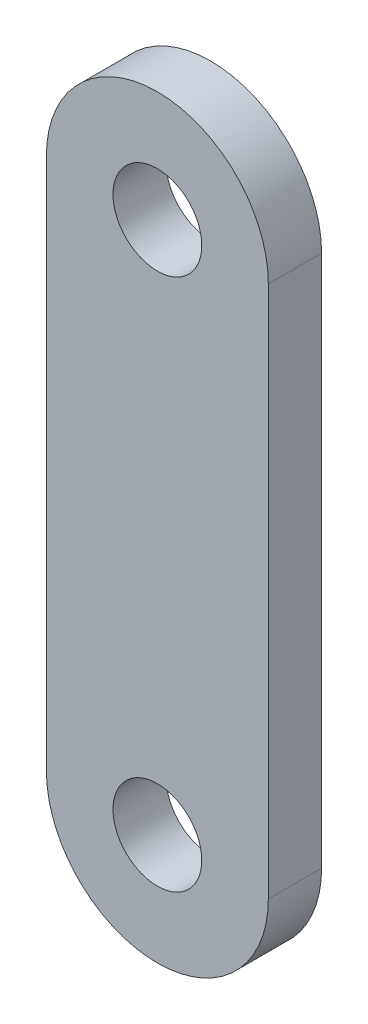
SolidWorks part; units mm, degrees
material "AISI 304"
ref_plane "Front Plane" through (0, 0, 0) normal (0, 0, 1) x (1, 0, 0)
ref_plane "Top Plane" through (0, 0, 0) normal (0, 1, 0) x (1, 0, 0)
ref_plane "Right Plane" through (0, 0, 0) normal (1, 0, 0) x (0, 0, -1)
other "Configuration Table"
sketch "Sketch1" plane through (0, 0, 0) normal (0, 0, 1) x (1, 0, 0)
  line L0 (0, 0) -> (0, 60) construction
  line L1 (-12.5, 0) -> (-12.5, 60)
  line L2 (12.5, 0) -> (12.5, 60)
  circle A0 centre (0, 0) radius 5
  arc A2 (-12.5, 0) -> (12.5, 0) centre (0, 0) ccw
  arc A3 (12.5, 60) -> (-12.5, 60) centre (0, 60) ccw
  circle A4 centre (0, 60) radius 5
  point P3 (0, 30)
  dimension "D1" = 10
  dimension "D2" = 60
  dimension "D3" = 12.5
  dimension "D4" = 10
extrude "Boss-Extrude1" add sketch "Sketch1" along normal mid plane 6
